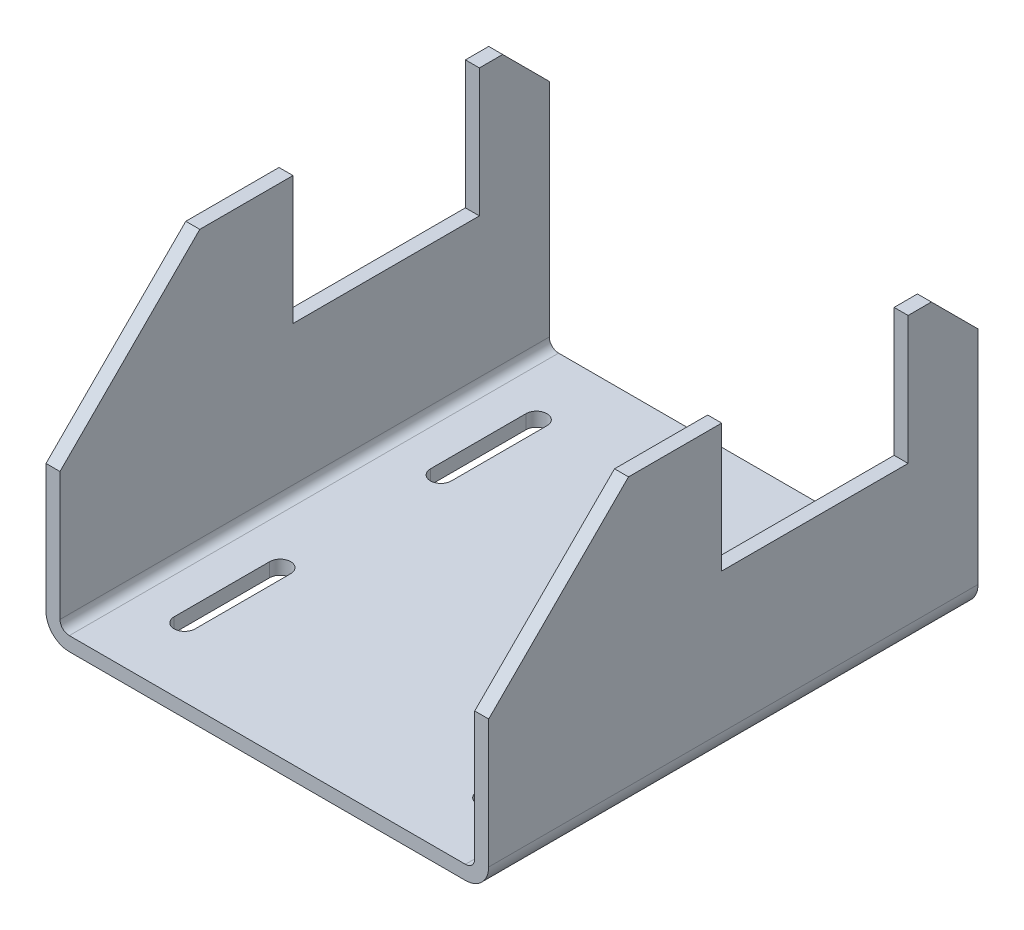
SolidWorks part; units mm, degrees
ref_plane "前视基准面" through (0, 0, 0) normal (0, 0, 1) x (1, 0, 0)
ref_plane "上视基准面" through (0, 0, 0) normal (0, 1, 0) x (1, 0, 0)
ref_plane "右视基准面" through (0, 0, 0) normal (1, 0, 0) x (0, 0, -1)
sketch "草图1" plane through (0, 0, 0) normal (0, 0, 1) x (1, 0, 0)
  line L0 (0, 0) -> (0, -115)
  line L1 (10, -125) -> (180, -125)
  line L2 (190, -115) -> (190, 0)
  line L3 (6, 0) -> (6, -115)
  line L4 (10, -119) -> (180, -119)
  line L5 (184, -115) -> (184, 0)
  line L6 (6, 0) -> (0, 0)
  line L7 (190, 0) -> (184, 0)
  arc A0 (180, -125) -> (190, -115) centre (180, -115) ccw
  arc A1 (0, -115) -> (10, -125) centre (10, -115) ccw
  arc A2 (6, -115) -> (10, -119) centre (10, -115) ccw
  arc A3 (180, -119) -> (184, -115) centre (180, -115) ccw
  point P7 (190, -125)
  point P10 (0, -125)
  dimension "D3" = 10
  dimension "D1" = 125
  dimension "D2" = 190
  dimension "D4" = 115
  dimension "D5" = 6
extrude "凸台-拉伸1" add sketch "草图1" along normal blind 210
chamfer "倒角1" distance 60 angle 45 2 edges at (187, 0, 210) (3, 0, 210)
chamfer "倒角2" distance 20 angle 45 2 edges at (3, 0, 0) (187, 0, 0)
sketch "草图3" plane through (0, -125, 0) normal (0, -1, 0) x (1, 0, 0)
  line L0 (30, 180.5) -> (30, 139.5) construction
  line L1 (34.5, 180.5) -> (34.5, 139.5)
  line L2 (25.5, 180.5) -> (25.5, 139.5)
  line L3 (160, 180.5) -> (160, 139.5) construction
  line L4 (164.5, 180.5) -> (164.5, 139.5)
  line L5 (155.5, 180.5) -> (155.5, 139.5)
  line L6 (30, 70.5) -> (30, 29.5) construction
  line L7 (34.5, 70.5) -> (34.5, 29.5)
  line L8 (25.5, 70.5) -> (25.5, 29.5)
  line L9 (160, 70.5) -> (160, 29.5) construction
  line L10 (164.5, 70.5) -> (164.5, 29.5)
  line L11 (155.5, 70.5) -> (155.5, 29.5)
  line L13 (10, 210) -> (180, 210) construction
  arc A0 (34.5, 180.5) -> (25.5, 180.5) centre (30, 180.5) ccw
  arc A1 (25.5, 139.5) -> (34.5, 139.5) centre (30, 139.5) ccw
  arc A2 (164.5, 180.5) -> (155.5, 180.5) centre (160, 180.5) ccw
  arc A3 (155.5, 139.5) -> (164.5, 139.5) centre (160, 139.5) ccw
  arc A4 (34.5, 70.5) -> (25.5, 70.5) centre (30, 70.5) ccw
  arc A5 (25.5, 29.5) -> (34.5, 29.5) centre (30, 29.5) ccw
  arc A6 (164.5, 70.5) -> (155.5, 70.5) centre (160, 70.5) ccw
  arc A7 (155.5, 29.5) -> (164.5, 29.5) centre (160, 29.5) ccw
  point P2 (30, 160)
  point P7 (160, 160)
  point P14 (30, 50)
  point P21 (160, 50)
  point P32 (95, 210)
  dimension "D2" = 69
  dimension "D3" = 130
  dimension "D4" = 65
  dimension "D5" = 29.5
  dimension "D6" = 4.5
  dimension "D1" = 41
extrude "切除-拉伸1" cut sketch "草图3" against normal blind 417
sketch "草图4" plane through (190, 0, 0) normal (1, 0, 0) x (0, 0, -1)
  line L0 (-150, 0) -> (-20, 0) construction
  line L1 (-30, -55) -> (-110, -55)
  line L2 (-30, -55) -> (-30, 35.776)
  line L3 (-30, 35.776) -> (-110, 35.776)
  line L4 (-110, -55) -> (-110, 35.776)
  line L5 (-30, -55) -> (-110, 35.776) construction
  line L6 (-30, 35.776) -> (-110, -55) construction
  line L7 (-210, -115) -> (-210, -60) construction
  point P0 (-70, -9.612)
  dimension "D1" = 80
  dimension "D2" = 55
  dimension "D3" = 100
extrude "切除-拉伸2" cut sketch "草图4" against normal blind 269
